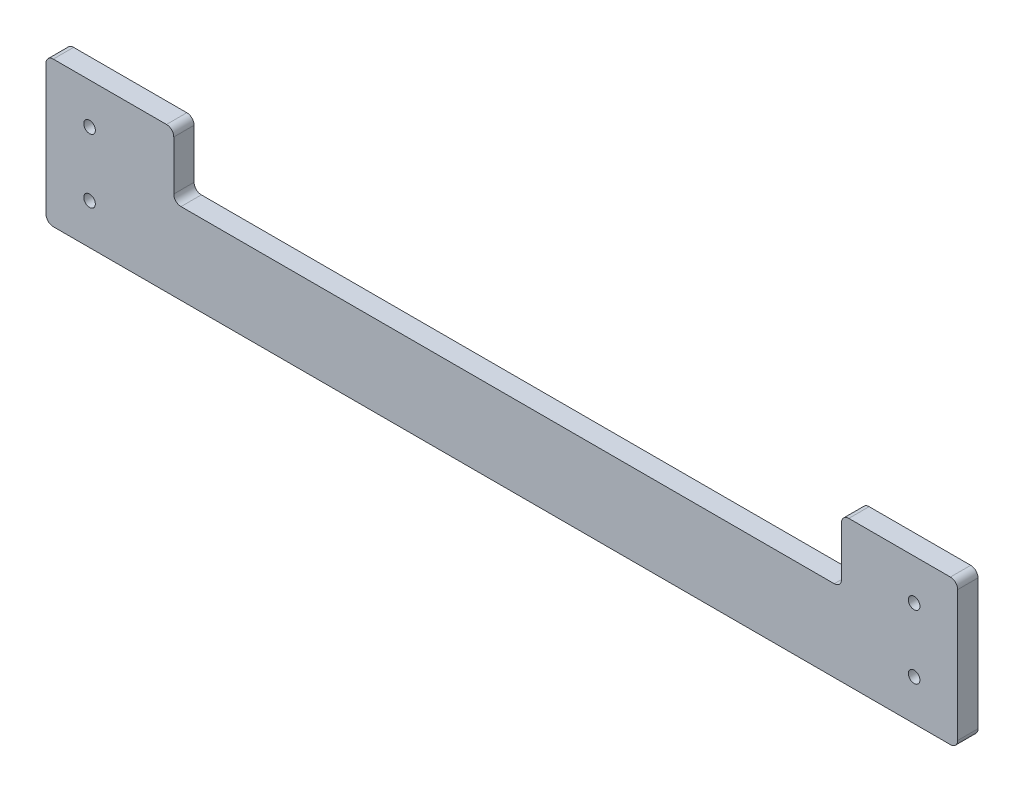
SolidWorks part; units mm, degrees
ref_plane "前视基准面" through (0, 0, 0) normal (0, 0, 1) x (1, 0, 0)
ref_plane "上视基准面" through (0, 0, 0) normal (0, 1, 0) x (1, 0, 0)
ref_plane "右视基准面" through (0, 0, 0) normal (1, 0, 0) x (0, 0, -1)
other "Configuration Table"
sketch "草图1" plane through (0, 0, 0) normal (0, 0, 1) x (1, 0, 0)
  line L1 (-785, -125) -> (785, -125)
  line L2 (-785, -125) -> (-785, 125)
  line L3 (-785, 125) -> (785, 125)
  line L4 (785, -125) -> (785, 125)
  line L5 (0, 125) -> (0, -125) construction
  line L6 (-785, 0) -> (785, 0) construction
  point P0 (0, 0)
  dimension "D1" = 1570
  dimension "D2" = 250
extrude "凸台-拉伸1" add sketch "草图1" along normal blind 35
sketch "草图2" plane through (0, 0, 35) normal (0, 0, 1) x (1, 0, 0)
  line L0 (-565, 125) -> (-565, 15)
  line L1 (785, 125) -> (-785, 125) construction
  line L2 (-565, 15) -> (585, 15)
  line L3 (585, 15) -> (585, 125)
  line L4 (585, 125) -> (-565, 125)
  line L5 (-785, 125) -> (-785, -125) construction
  line L6 (785, -125) -> (785, 125) construction
  dimension "D1" = 220
  dimension "D3" = 200
  dimension "D4" = 110
extrude "切除-拉伸1" cut sketch "草图2" against normal up to next
fillet "圆角1" radius 12.5 8 edges at (-565, 15, 17.5) (-565, 125, 17.5) (585, 15, 17.5) (585, 125, 17.5) (785, 125, 17.5) (785, -125, 17.5) (-785, -125, 17.5) (-785, 125, 17.5)
sketch "草图4" plane through (0, 0, 35) normal (0, 0, 1) x (1, 0, 0)
  line L0 (785, -112.5) -> (785, 112.5) construction
  line L1 (-785, 0) -> (785, 0) construction
  line L2 (-785, 112.5) -> (-785, -112.5) construction
  circle A0 centre (-710, 55) radius 10
  circle A1 centre (-710, -55) radius 10
  circle A2 centre (710, 55) radius 10
  circle A3 centre (710, -55) radius 10
  dimension "D1" = 20
  dimension "D2" = 20
  dimension "D10" = 20
  dimension "D11" = 20
  dimension "D12" = 55
  dimension "D3" = 75
  dimension "D4" = 75
  dimension "D5" = 110
  dimension "D6" = 55
  dimension "D7" = 55
  dimension "D8" = 75
  dimension "D9" = 75
extrude "切除-拉伸2" cut sketch "草图4" against normal up to next
